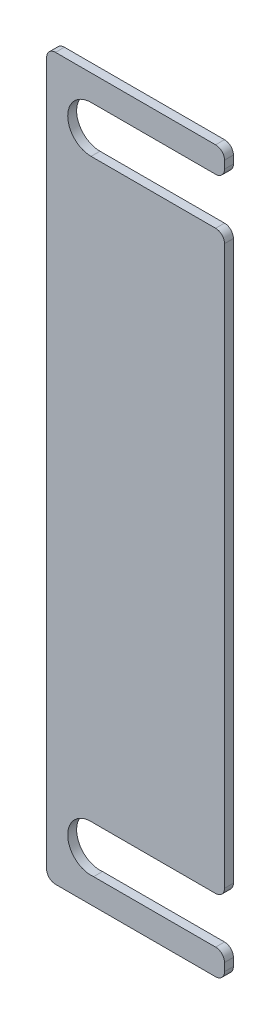
from build123d import *

# Parameters (mm, degrees)
SKETCH_1_W          = 40
SKETCH_1_H          = 162
EXTRUDE_1_DEPTH     = 2
SKETCH_2_R          = 5.25
CUT_EXTRUDE_1_DEPTH = 3
SKETCH_4_W          = 30
SKETCH_4_H          = 10.5
SKETCH_4_W_2        = 29.434352085
SKETCH_4_H_2        = 10.438877802
CUT_EXTRUDE_4_DEPTH = 10
FILLET_2_R          = 2


with BuildPart() as part:
    # 草图1 → 凸台-拉伸1 (new body)
    with BuildSketch(Plane.XY):
        Rectangle(SKETCH_1_W, SKETCH_1_H)
    extrude(amount=EXTRUDE_1_DEPTH)

    # 草图2 → 切除-拉伸1 (cut)
    with BuildSketch(Plane.XY.offset(2)):
        with Locations((-10, 70)):
            Circle(SKETCH_2_R)
        with Locations((-10, -70)):
            Circle(SKETCH_2_R)
    extrude(amount=-CUT_EXTRUDE_1_DEPTH, mode=Mode.SUBTRACT)

    # 草图4 → 切除-拉伸4 (cut)
    with BuildSketch(Plane.XY.offset(2)):
        with Locations((5, 70)):
            Rectangle(SKETCH_4_W, SKETCH_4_H)
        with Locations((5.282823957, -70)):
            Rectangle(SKETCH_4_W_2, SKETCH_4_H_2)
    extrude(amount=-CUT_EXTRUDE_4_DEPTH, mode=Mode.SUBTRACT)

    # 圆角2
    fillet_2_edges = [part.edges().sort_by_distance(p)[0] for p in [
        (20, 75.25, 1),
        (20, 64.75, 1),
        (20, -64.780561099, 1),
        (20, -75.219438901, 1),
        (-20, 81, 1),
        (20, 81, 1),
        (20, -81, 1),
        (-20, -81, 1),
    ]]
    fillet(fillet_2_edges, radius=FILLET_2_R)


solid = part.part
